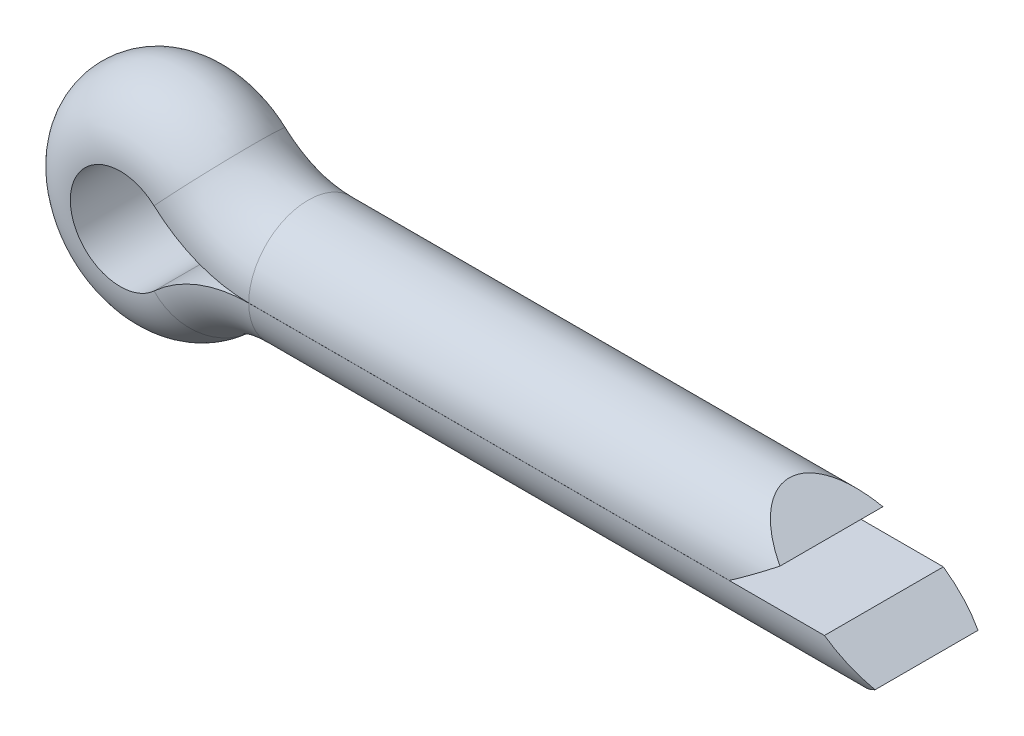
from build123d import *

# Parameters (mm, degrees)
CONECUT_DEPTH      = 27.521877713
CONECUT_DEPTH_BACK = 27.521877713


with BuildPart() as part:
    # Body: sweep along a path in Sketch2
    with BuildLine(Plane.XY) as body_path:
        Line((22, 2.5), (0, 2.5))
        ThreePointArc((0, 2.5), (-1.229728386, 2.730698436), (-2.292225201, 3.391420912))
        ThreePointArc((-2.292225201, 3.391420912), (-10, 0), (-2.292225201, -3.391420912))
        ThreePointArc((-2.292225201, -3.391420912), (-1.229728386, -2.730698436), (0, -2.5))
        Line((0, -2.5), (26, -2.5))
    # Sketch1 → Body (sweep)
    with BuildSketch(Plane(origin=(22, 0, 0), x_dir=(0, 0, -1), z_dir=(1, 0, 0))):
        with BuildLine():
            Line((-2.4999992, 0.002), (2.4999992, 0.002))
            ThreePointArc((2.4999992, 0.002), (0, 2.5), (-2.4999992, 0.002))
        make_face()
    sweep(path=body_path.line)

    # Sketch3 → ConeCut (cut, two sides: drawn at the far end of the back side and taken through both)
    with BuildSketch(Plane.XY.offset(-CONECUT_DEPTH_BACK)):
        Polygon((22, 1.251), (20.210475082, 2.51), (26.01, 2.51), (26.01, -2.51), (24.210475082, -2.51), (26, -1.251), (24.204873421, 0), (20.204873421, 0), align=None)
    extrude(amount=CONECUT_DEPTH + CONECUT_DEPTH_BACK, mode=Mode.SUBTRACT)


solid = part.part
